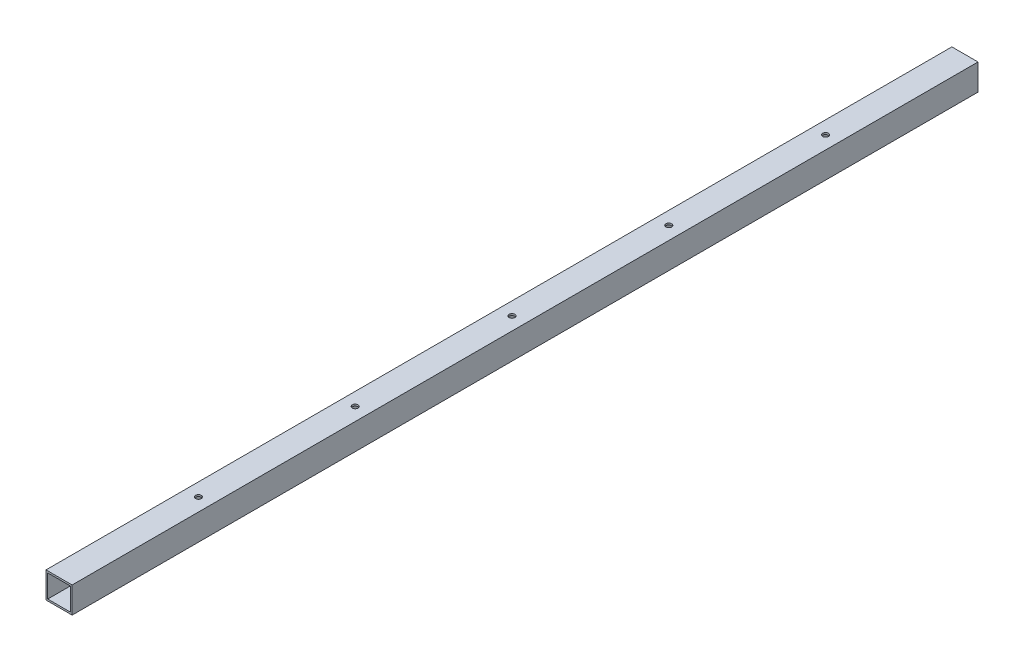
SolidWorks part; units mm, degrees
ref_plane "前视基准面" through (0, 0, 0) normal (0, 0, 1) x (1, 0, 0)
ref_plane "上视基准面" through (0, 0, 0) normal (0, 1, 0) x (1, 0, 0)
ref_plane "右视基准面" through (0, 0, 0) normal (1, 0, 0) x (0, 0, -1)
sketch "草图1" plane through (0, 0, 0) normal (0, 0, 1) x (1, 0, 0)
  line L0 (13, 13) -> (-13, 13)
  line L1 (15, -15) -> (-15, -15)
  line L2 (15, -15) -> (15, 15)
  line L3 (15, 15) -> (-15, 15)
  line L4 (-15, -15) -> (-15, 15)
  line L5 (15, -15) -> (-15, 15) construction
  line L6 (15, 15) -> (-15, -15) construction
  line L7 (-13, -13) -> (-13, 13)
  line L8 (13, -13) -> (-13, -13)
  line L9 (13, -13) -> (13, 13)
  point P0 (0, 0)
  dimension "D1" = 30
  dimension "D2" = 2
extrude "凸台-拉伸1" add sketch "草图1" along normal mid plane 1040
sketch "草图2" plane through (0, 0, 520) normal (0, 0, 1) x (1, 0, 0)
  circle A1 centre (0, 0) radius 10.0238
sketch "草图3" plane through (0, 15, 0) normal (0, 1, 0) x (1, 0, 0)
  line L0 (0, 360) -> (0, 180) construction
  line L1 (0, 180) -> (0, 0) construction
  line L2 (0, 0) -> (0, -180) construction
  line L4 (0, -180) -> (0, -360) construction
  circle A0 centre (0, 360) radius 3.3
  circle A1 centre (0, 180) radius 3.3
  circle A2 centre (0, 0) radius 3.3
  circle A3 centre (0, -180) radius 3.3
  circle A4 centre (0, -360) radius 3.3
  dimension "D2" = 6.6
  dimension "D1" = 180
extrude "切除-拉伸1" cut sketch "草图3" against normal blind 636
